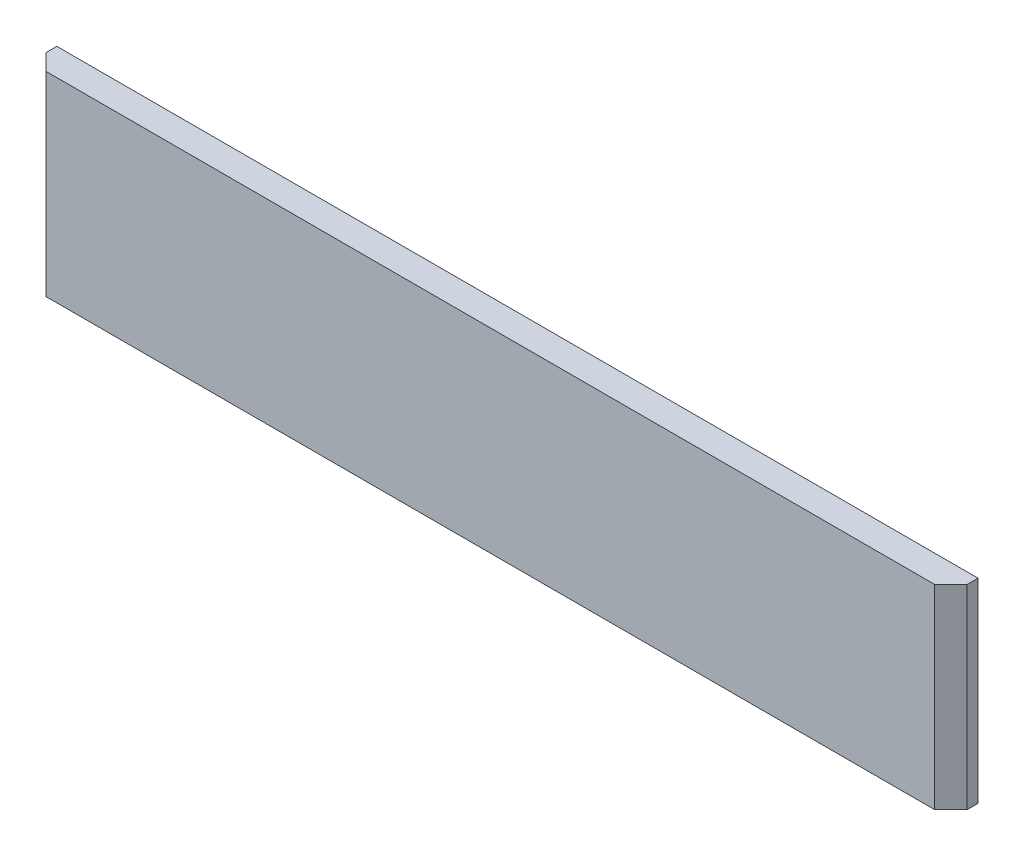
SolidWorks part; units mm, degrees
material "Q235-A"
ref_plane "Front Plane" through (0, 0, 0) normal (0, 0, 1) x (1, 0, 0)
ref_plane "Top Plane" through (0, 0, 0) normal (0, 1, 0) x (1, 0, 0)
ref_plane "Right Plane" through (0, 0, 0) normal (1, 0, 0) x (0, 0, -1)
sketch "Sketch1" plane through (0, 0, 0) normal (0, 0, 1) x (1, 0, 0)
  line L1 (425, -90) -> (-425, -90)
  line L2 (425, -90) -> (425, 90)
  line L3 (425, 90) -> (-425, 90)
  line L4 (-425, -90) -> (-425, 90)
  line L5 (425, -90) -> (-425, 90) construction
  line L6 (425, 90) -> (-425, -90) construction
  point P0 (0, 0)
  dimension "D1" = 850
  dimension "D2" = 180
extrude "Boss-Extrude1" add sketch "Sketch1" along normal mid plane 40
chamfer "Chamfer1" distance 15 angle 45 6 edges at (0, -90, -20) (425, 0, -20) (0, 90, -20) (-425, 0, -20) (425, 0, 20) (-425, 0, 20)
